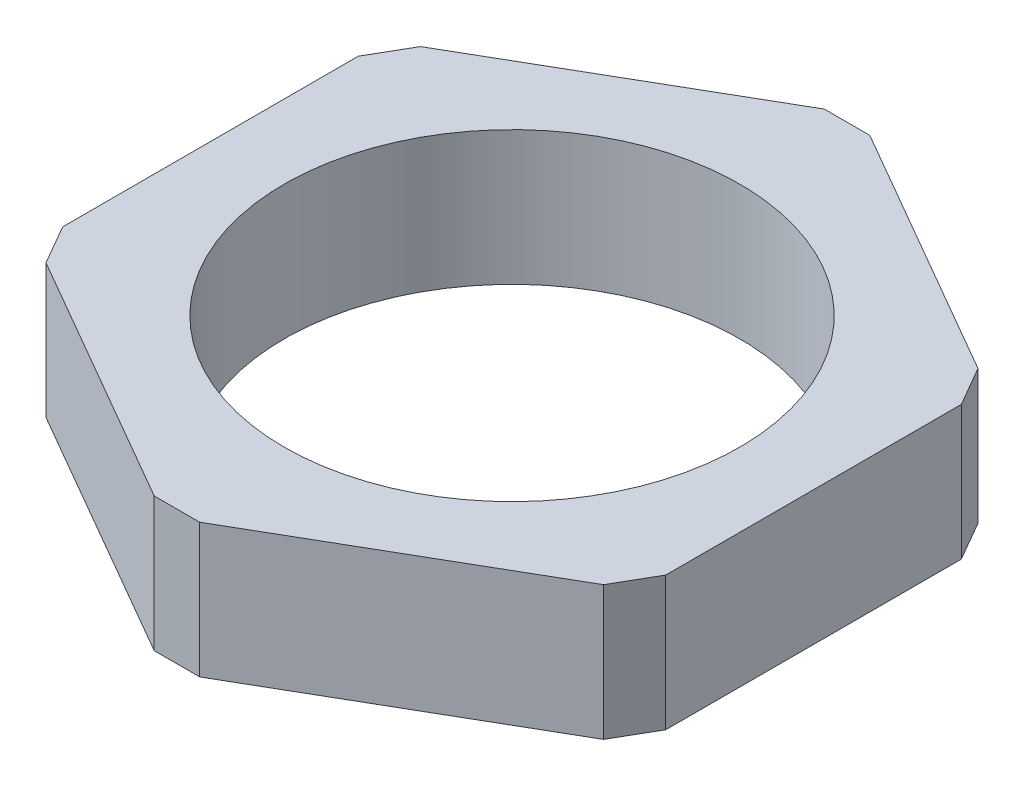
SolidWorks part; units mm, degrees
ref_plane "Front Plane" through (0, 0, 0) normal (0, 0, 1) x (1, 0, 0)
ref_plane "Top Plane" through (0, 0, 0) normal (0, 1, 0) x (1, 0, 0)
ref_plane "Right Plane" through (0, 0, 0) normal (1, 0, 0) x (0, 0, -1)
other "Configuration Table"
sketch "Sketch1" plane through (0, 0, 0) normal (0, 1, 0) x (1, 0, 0)
  line L1 (22.5, -12.9904) -> (22.5, 12.9904)
  line L2 (22.5, 12.9904) -> (0, 25.9808)
  line L3 (0, 25.9808) -> (-22.5, 12.9904)
  line L4 (-22.5, 12.9904) -> (-22.5, -12.9904)
  line L5 (-22.5, -12.9904) -> (0, -25.9808)
  line L6 (0, -25.9808) -> (22.5, -12.9904)
  circle A0 centre (0, 0) radius 22.5 construction
  dimension "D1" = 45
extrude "Boss-Extrude1" add sketch "Sketch1" along normal blind 10
hole_wizard "M36x2.0 Tapped Hole1" positions "Sketch2" profile "Sketch3" tap size "M36x2.0" standard "GB"
sketch "Sketch2" plane through (0, 10, 0) normal (0, 1, 0) x (1, 0, 0)
  point P0 (0, 0)
sketch "Sketch3" plane through (0, 10, 0) normal (1, 0, 0) x (0, 0, 1)
  line L0 (0, 0) -> (0, 92.2146)
  line L1 (0, 92.2146) -> (17, 82)
  line L2 (17, 82) -> (17, 0)
  line L5 (17, 0) -> (0, 0)
  line L10 (0, 92.2146) -> (-17, 82) construction
  line L11 (0, -6.35) -> (0, 107.95) construction
  dimension "螺纹孔钻头直径" = 34
  dimension "螺纹孔钻头深度" = 82
  dimension "导头角度" = 118
cosmetic thread "Hole Thread Line1" parameters "D1"=72, "D2"=36
sketch "Sketch4" plane through (0, 10, 0) normal (0, 1, 0) x (1, 0, 0)
  line L1 (-8.2414, 32.8699) -> (11.0681, 32.8699)
  line L2 (-8.2414, 32.8699) -> (-8.2414, 25)
  line L3 (-8.2414, 25) -> (11.0681, 25)
  line L4 (11.0681, 32.8699) -> (11.0681, 25)
  line L5 (-8.2414, 32.8699) -> (11.0681, 25) construction
  line L6 (-8.2414, 25) -> (11.0681, 32.8699) construction
  point P0 (1.4133, 28.9349)
  dimension "D1" = 25
extrude "Cut-Extrude1" cut sketch "Sketch4" against normal blind 88
pattern_circular "CirPattern1" count 6 over 360 about axis through (0, 0, 0) along (0, 1, 0) of "Cut-Extrude1"
